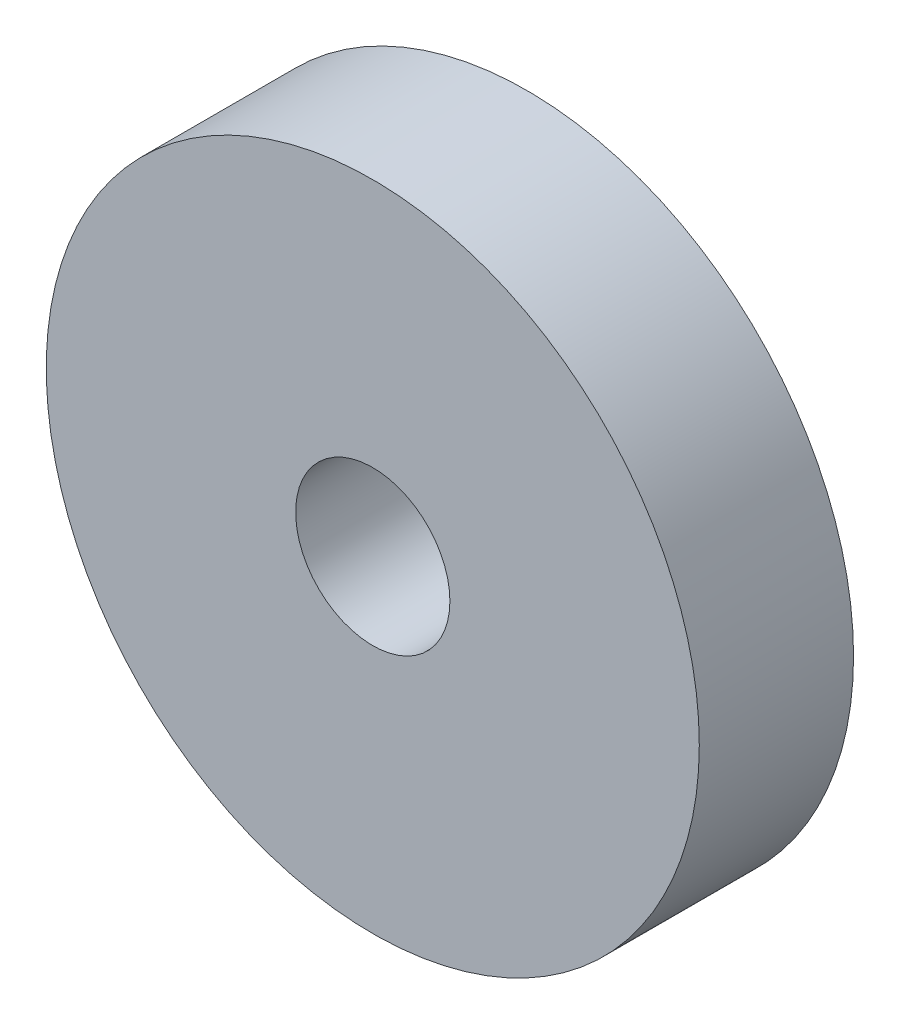
from build123d import *

# Parameters (mm, degrees)
SKETCH1_R           = 12.7
SKETCH1_R_2         = 3
BOSS_EXTRUDE1_DEPTH = 6


with BuildPart() as part:
    # Sketch1 → Boss-Extrude1 (new body)
    with BuildSketch(Plane.XY):
        Circle(SKETCH1_R)
        Circle(SKETCH1_R_2, mode=Mode.SUBTRACT)
    extrude(amount=BOSS_EXTRUDE1_DEPTH)


solid = part.part
